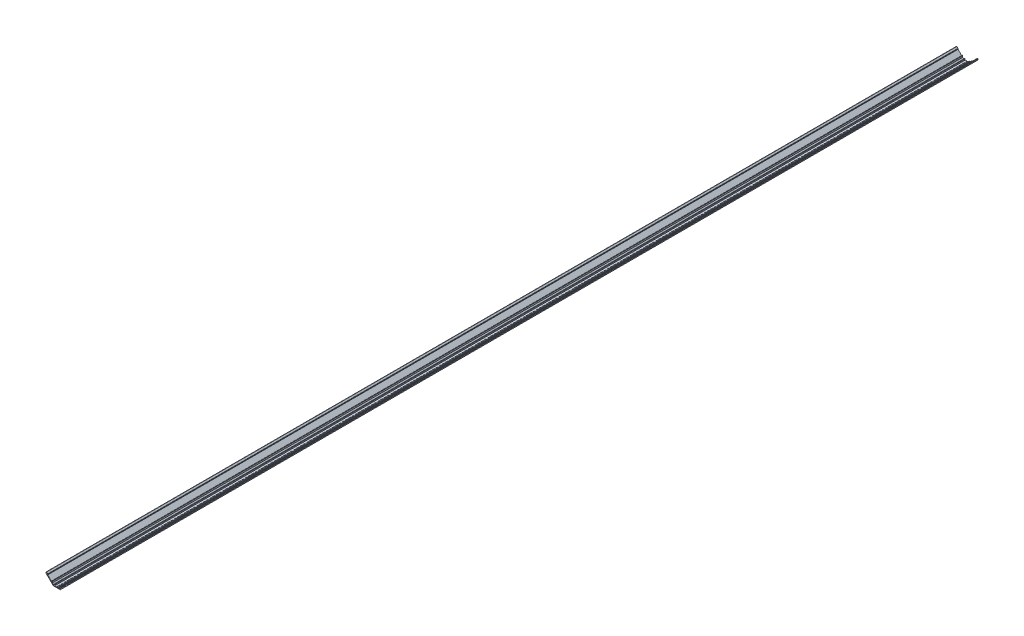
from build123d import *

# Parameters (mm, degrees)
EXTRUDE_1_DEPTH = 1192.5


with BuildPart() as part:
    # 草图2 → 凸台-拉伸1 (new, symmetric)
    with BuildSketch(Plane.XY):
        with BuildLine():
            Line((6.75, 5), (5.25, 5))
            Line((5.25, 5), (5.25, 2))
            Line((5.25, 2), (0.25, 2))
            ThreePointArc((0.25, 2), (0, 1.75), (-0.25, 2))
            Line((-0.25, 2), (-5.25, 2))
            Line((-5.25, 2), (-5.25, 5))
            Line((-5.25, 5), (-6.75, 5))
            Line((-6.75, 5), (-6.75, 2))
            Line((-6.75, 2), (-8.634653896, 2))
            Line((-8.634653896, 2), (-11.75, 5.119363474))
            Line((-11.75, 5.119363474), (-11.75, 8.88650173))
            Line((-11.75, 8.88650173), (-12.25, 9.38650173))
            Line((-12.25, 9.38650173), (-12.75, 9.38650173))
            Line((-12.75, 9.38650173), (-12.75, 7.328070483))
            ThreePointArc((-12.75, 7.328070483), (-13.058886266, 6.866036349), (-13.603902163, 6.97486621))
            Line((-13.603902163, 6.97486621), (-23.891097866, 17.282388203))
            Line((-23.891097866, 17.282388203), (-23.891097866, 19.37637924))
            Line((-23.891097866, 19.37637924), (-26.873078382, 22.358359756))
            Line((-26.873078382, 22.358359756), (-27.580185163, 22.358359756))
            Line((-27.580185163, 22.358359756), (-28.284271248, 21.654273671))
            Line((-28.284271248, 21.654273671), (-28.284271248, 19.102647866))
            Line((-28.284271248, 19.102647866), (-9.181623382, 0))
            Line((-9.181623382, 0), (9.181623382, 0))
            Line((9.181623382, 0), (28.287291944, 19.105668562))
            Line((28.287291944, 19.105668562), (28.287291944, 21.651252975))
            Line((28.287291944, 21.651252975), (27.580185163, 22.358359756))
            Line((27.580185163, 22.358359756), (26.873078382, 22.358359756))
            Line((26.873078382, 22.358359756), (23.891097866, 19.376379241))
            Line((23.891097866, 19.376379241), (23.891097866, 17.282388203))
            Line((23.891097866, 17.282388203), (13.603902163, 6.97486621))
            ThreePointArc((13.603902163, 6.97486621), (13.058886266, 6.866036349), (12.75, 7.328070483))
            Line((12.75, 7.328070483), (12.75, 9.38650173))
            Line((12.75, 9.38650173), (12.25, 9.38650173))
            Line((12.25, 9.38650173), (11.75, 8.88650173))
            Line((11.75, 8.88650173), (11.75, 5.118657708))
            Line((11.75, 5.118657708), (8.636038969, 2))
            Line((8.636038969, 2), (6.75, 2))
            Line((6.75, 2), (6.75, 5))
        make_face()
    extrude(amount=EXTRUDE_1_DEPTH, both=True)


solid = part.part
